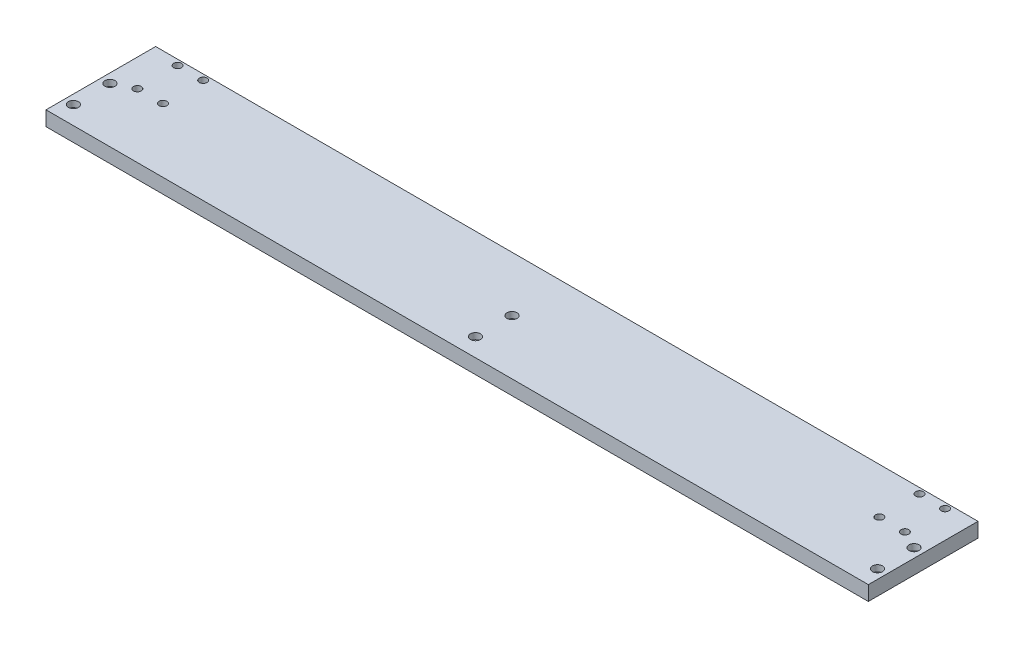
from build123d import *

# Parameters (mm, degrees)
SKETCH_1_W                = 900
SKETCH_1_H                = 120
EXTRUDE_1_DEPTH           = 16
HOLE_WIZARD_8_5_8_5_1_D   = 8.5
HOLE_WIZARD_1_D           = 6.6
HOLE_WIZARD_1_CBORE_D     = 11
HOLE_WIZARD_1_CBORE_DEPTH = 6.8
PATTERN_LINEAR_1_COUNT    = 3
PATTERN_LINEAR_1_PITCH    = 440


with BuildPart() as part:
    # 草图1 → 凸台-拉伸1 (new body)
    with BuildSketch(Plane(origin=(0, 0, 0), x_dir=(1, 0, 0), z_dir=(0, 1, 0))):
        Rectangle(SKETCH_1_W, SKETCH_1_H)
    extrude(amount=EXTRUDE_1_DEPTH)

    # Ø8.5 (8.5) 直径孔1 (through all)
    with Locations(Plane(origin=(0, 16, 0), x_dir=(1, 0, 0), z_dir=(0, 1, 0))):
        with Locations((392, 54), (420, 54), (392, 10), (420, 10)):
            hole_wizard_8_5_8_5_1 = Hole(HOLE_WIZARD_8_5_8_5_1_D / 2)

    # 打孔尺寸(%根据)内六角圆柱头螺钉的类型1 (through all)
    with Locations(Plane(origin=(0, 16, 0), x_dir=(1, 0, 0), z_dir=(0, 1, 0))):
        with Locations((-440, 0), (-440, -40)):
            hole_wizard_1 = CounterBoreHole(HOLE_WIZARD_1_D / 2, HOLE_WIZARD_1_CBORE_D / 2, HOLE_WIZARD_1_CBORE_DEPTH)

    # 阵列(线性)1: 打孔尺寸(%根据)内六角圆柱头螺钉的类型1 ×3
    with Locations(*[(i * PATTERN_LINEAR_1_PITCH, 0, 0) for i in range(1, PATTERN_LINEAR_1_COUNT)]):
        add(hole_wizard_1, mode=Mode.SUBTRACT)

    # 镜向1: Ø8.5 (8.5) 直径孔1 across plane
    add(hole_wizard_8_5_8_5_1.mirror(Plane(origin=(0, 0, 0), x_dir=(0, 0, 1), z_dir=(1, 0, 0))), mode=Mode.SUBTRACT)


solid = part.part
